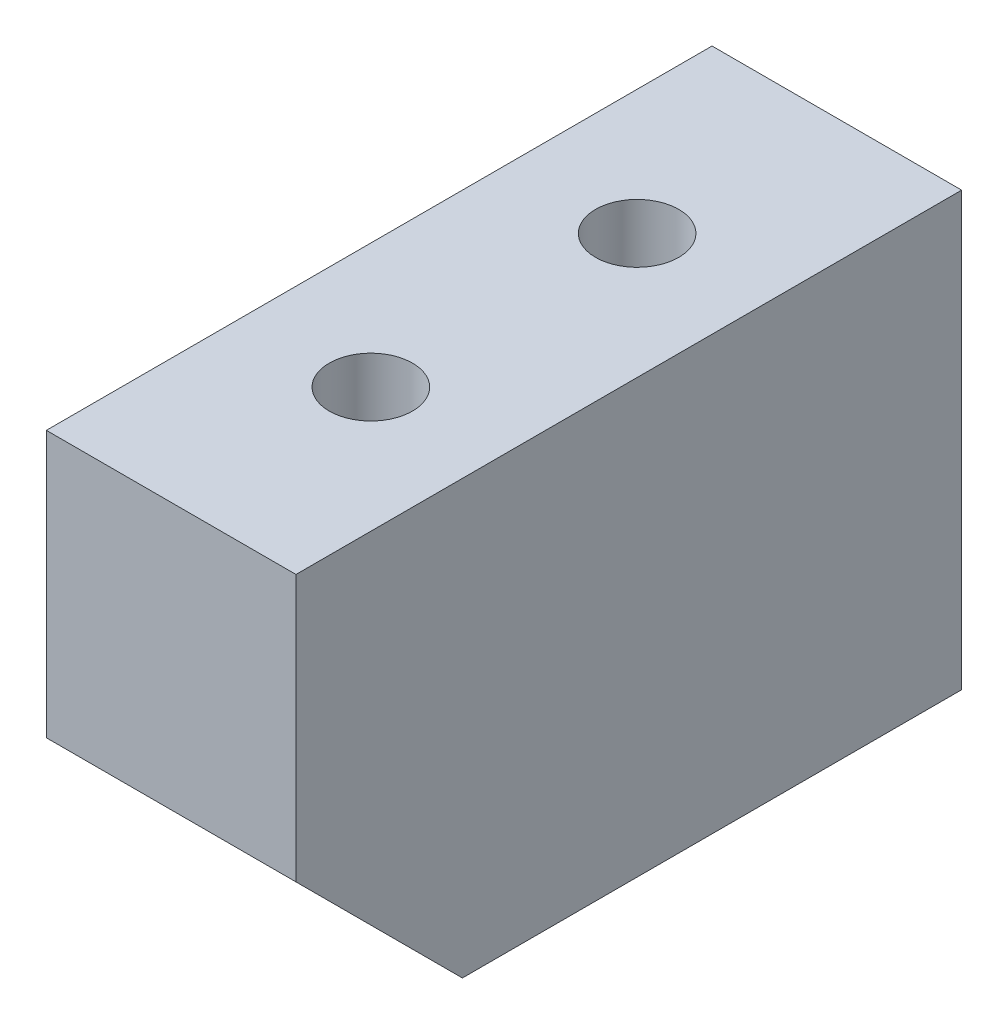
from build123d import *

# Parameters (mm, degrees)
SKETCH_1_W             = 15
SKETCH_1_H             = 26
EXTRUDE_1_DEPTH        = 40
HOLE_WIZARD_M6_1_D     = 5
HOLE_WIZARD_M6_1_DEPTH = 15
HOLE_WIZARD_M6_1_TIP   = 1.502151548
HOLE_WIZARD_M6_2_D     = 5
HOLE_WIZARD_M6_2_DEPTH = 15
HOLE_WIZARD_M6_2_TIP   = 1.502151548
CHAMFER_2_SIZE         = 10


with BuildPart() as part:
    # 草图1 → 凸台-拉伸1 (new body)
    with BuildSketch(Plane.XY):
        Rectangle(SKETCH_1_W, SKETCH_1_H)
    extrude(amount=EXTRUDE_1_DEPTH)

    # M6 螺纹孔1
    with Locations(Plane(origin=(0, 13, 0), x_dir=(1, 0, 0), z_dir=(0, 1, 0))):
        with Locations((0, -12), (0, -28)):
            Hole(HOLE_WIZARD_M6_1_D / 2, depth=HOLE_WIZARD_M6_1_DEPTH)
            with Locations((0, 0, -(HOLE_WIZARD_M6_1_DEPTH + HOLE_WIZARD_M6_1_TIP / 2))):  # 118° drill point
                Cone(0, HOLE_WIZARD_M6_1_D / 2, HOLE_WIZARD_M6_1_TIP, mode=Mode.SUBTRACT)

    # M6 螺纹孔2
    with Locations(Plane(origin=(0, 0, 0), x_dir=(-1, 0, 0), z_dir=(0, 0, -1))):
        with Locations((0, 0)):
            Hole(HOLE_WIZARD_M6_2_D / 2, depth=HOLE_WIZARD_M6_2_DEPTH)
            with Locations((0, 0, -(HOLE_WIZARD_M6_2_DEPTH + HOLE_WIZARD_M6_2_TIP / 2))):  # 118° drill point
                Cone(0, HOLE_WIZARD_M6_2_D / 2, HOLE_WIZARD_M6_2_TIP, mode=Mode.SUBTRACT)

    # 倒角2
    chamfer_2_edges = [part.edges().sort_by_distance(p)[0] for p in [
        (0, -13, 40),
    ]]
    chamfer(chamfer_2_edges, length=CHAMFER_2_SIZE)


solid = part.part
